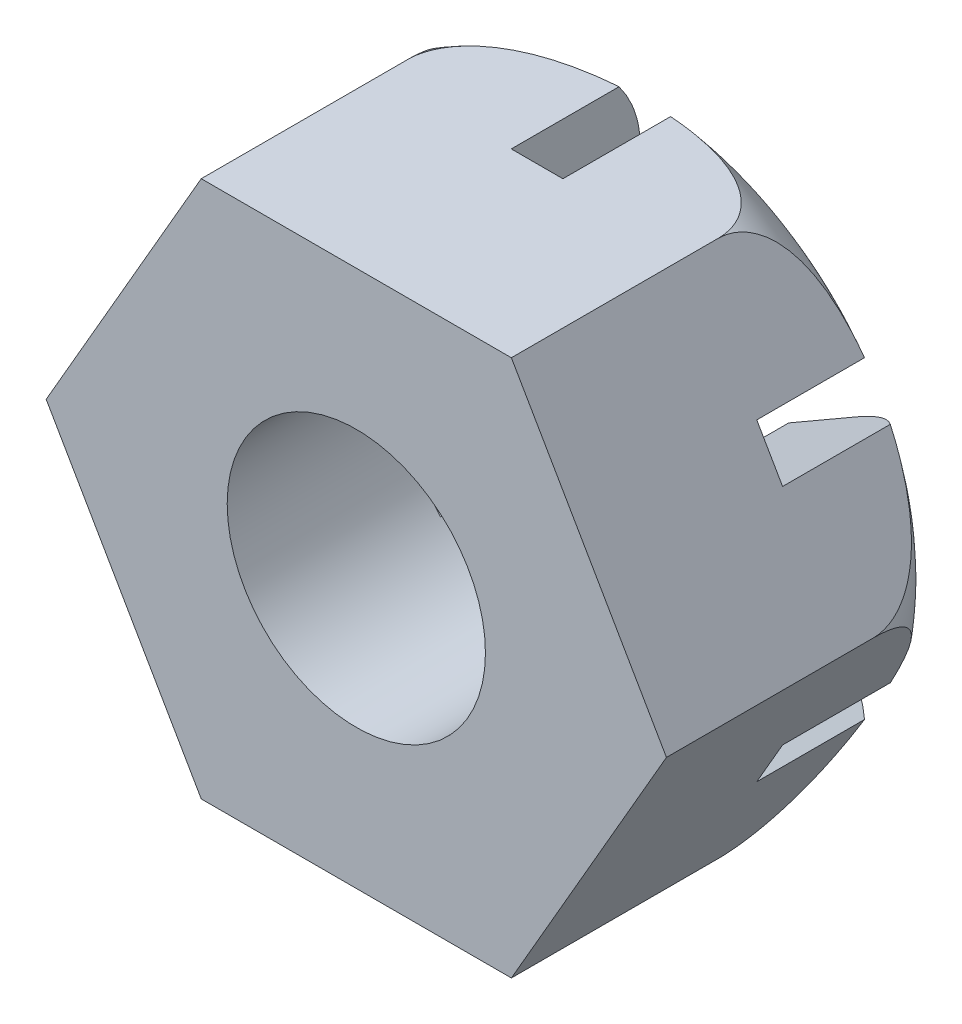
from build123d import *

# Parameters (mm, degrees)
BOSS_EXTRUDE1_DEPTH     = 60
SKETCH3_W               = 10
SKETCH3_H               = 25
CUT_EXTRUDE1_DEPTH      = 135.243559913
CIRPATTERN1_COUNT       = 6
CUT_EXTRUDE2_DEPTH      = 87.800537803
CUT_EXTRUDE2_DEPTH_BACK = 87.800537803
SKETCH4_R               = 25


with BuildPart() as part:
    # Sketch1 → Boss-Extrude1 (new body)
    with BuildSketch(Plane.XY):
        Polygon((30.022213998, -52), (60.044427996, 0), (30.022213998, 52), (-30.022213998, 52), (-60.044427996, 0), (-30.022213998, -52), align=None)
    extrude(amount=BOSS_EXTRUDE1_DEPTH)

    # Sketch2 → Cut-Revolve1 (revolve, cut)
    with BuildSketch(Plane(origin=(0, 0, 0), x_dir=(1, 0, 0), z_dir=(0, 1, 0))):
        with BuildLine():
            Line((-60.044427996, -20), (-60.044427996, 0))
            Line((-60.044427996, 0), (-40.044427996, 0))
            ThreePointArc((-40.044427996, 0), (-54.186563619, -5.857864376), (-60.044427996, -20))
        make_face()
    revolve(axis=Axis((0, 0, -15.505085141), (0, 0, 1)), mode=Mode.SUBTRACT)

    # Sketch3 → Cut-Extrude1 (cut, through all)
    with BuildSketch(Plane(origin=(0, 52, 0), x_dir=(1, 0, 0), z_dir=(0, 1, 0))):
        with Locations((0, -12.5)):
            Rectangle(SKETCH3_W, SKETCH3_H)
    cut_extrude1 = extrude(amount=-CUT_EXTRUDE1_DEPTH, mode=Mode.SUBTRACT)

    # CirPattern1: Cut-Extrude1 ×6 about axis
    cirpattern1_axis = Axis((0, 0, 0), (0, 0, 1))
    for i in range(1, CIRPATTERN1_COUNT):
        add(cut_extrude1.rotate(cirpattern1_axis, i * 360 / CIRPATTERN1_COUNT), mode=Mode.SUBTRACT)

    # Sketch4 → Cut-Extrude2 (cut, two sides: drawn at the far end of the back side and taken through both)
    with BuildSketch(Plane(origin=(0, 0, 25), x_dir=(-1, 0, 0), z_dir=(0, 0, -1)).offset(-CUT_EXTRUDE2_DEPTH_BACK)):
        with Locations(Location((0, 0, 0), (0, 0, 161.536959033))):
            Circle(SKETCH4_R)
    extrude(amount=CUT_EXTRUDE2_DEPTH + CUT_EXTRUDE2_DEPTH_BACK, mode=Mode.SUBTRACT)


solid = part.part
